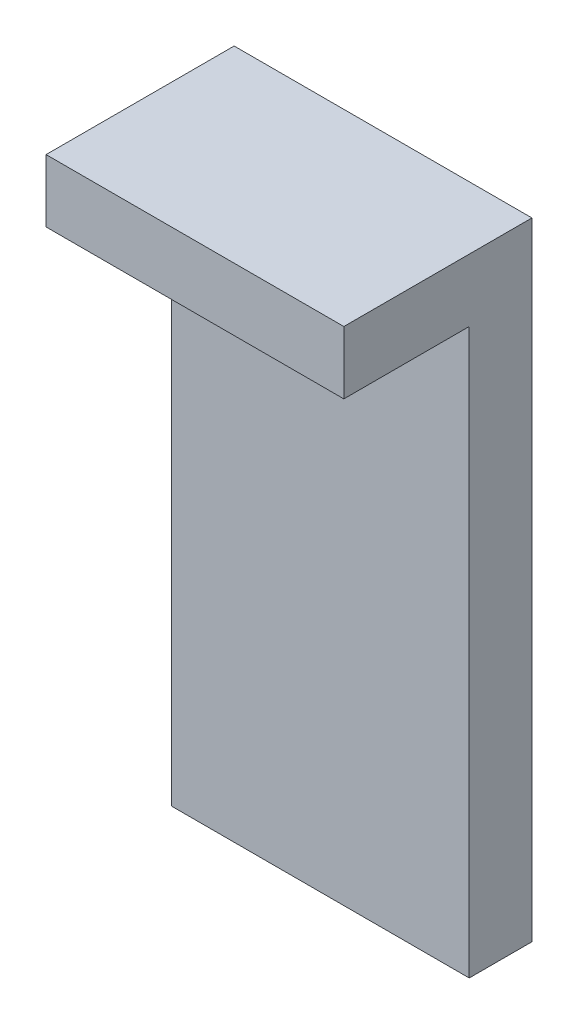
from build123d import *

# Parameters (mm, degrees)
SKETCH_1_W      = 38
SKETCH_1_H      = 80
EXTRUDE_1_DEPTH = 4
SKETCH_2_W      = 38
SKETCH_2_H      = 8
EXTRUDE_2_DEPTH = 16


with BuildPart() as part:
    # 草图1 → 凸台-拉伸1 (new, symmetric)
    with BuildSketch(Plane.XY):
        Rectangle(SKETCH_1_W, SKETCH_1_H)
    extrude(amount=EXTRUDE_1_DEPTH, both=True)

    # 草图2 → 凸台-拉伸2 (add)
    with BuildSketch(Plane.XY.offset(4)):
        with Locations((0, 36)):
            Rectangle(SKETCH_2_W, SKETCH_2_H)
    extrude(amount=EXTRUDE_2_DEPTH)


solid = part.part
